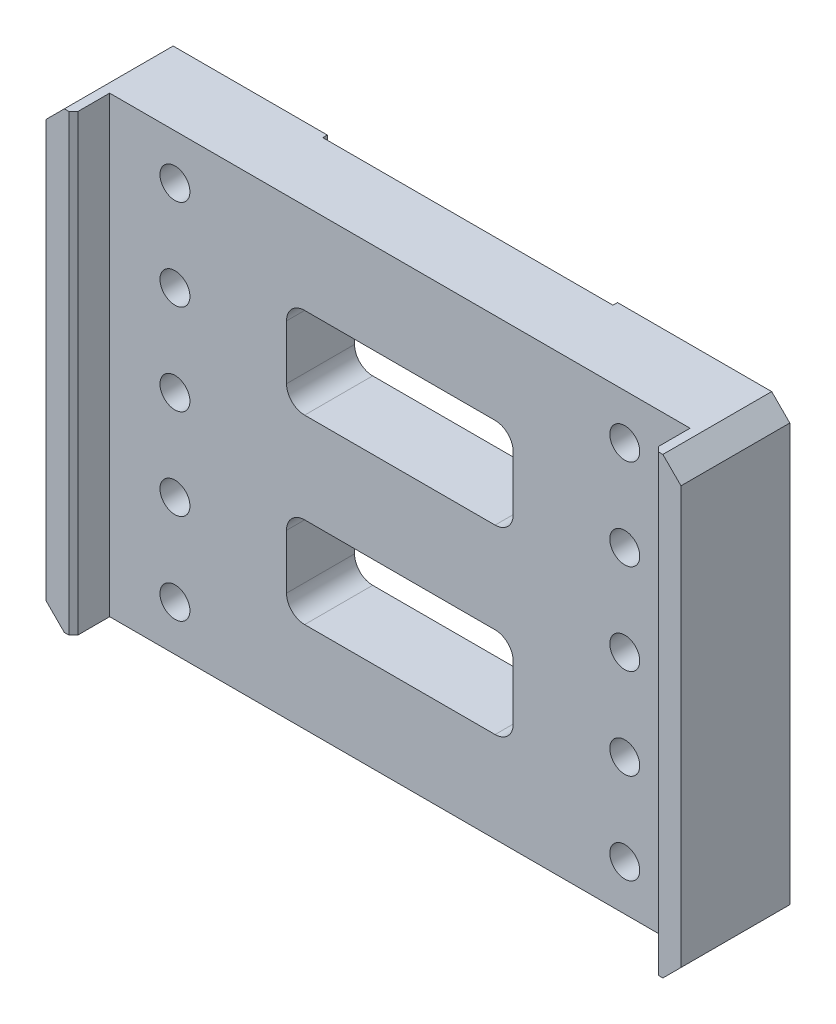
from build123d import *

# Parameters (mm, degrees)
SKETCH1_W           = 70
SKETCH1_H           = 50
BOSS_EXTRUDE1_DEPTH = 12
SKETCH2_W           = 64
SKETCH2_H           = 4
CUT_EXTRUDE1_DEPTH  = 63.20128616
CHAMFER1_SIZE       = 0.5
SKETCH3_W           = 32
SKETCH3_H           = 0.5
CUT_EXTRUDE2_DEPTH  = 63.20128616
LPATTERN1_COUNT     = 5
LPATTERN1_PITCH     = 10
SKETCH7_W           = 25
SKETCH7_H           = 10
CUT_EXTRUDE3_DEPTH  = 44.749285708
FILLET1_R           = 2
CHAMFER2_SIZE       = 2


with BuildPart() as part:
    # Sketch1 → Boss-Extrude1 (new body)
    with BuildSketch(Plane.XY):
        Rectangle(SKETCH1_W, SKETCH1_H)
    extrude(amount=BOSS_EXTRUDE1_DEPTH)

    # Sketch2 → Cut-Extrude1 (cut, through all)
    with BuildSketch(Plane.XZ.offset(25)):
        with Locations((0, 10)):
            Rectangle(SKETCH2_W, SKETCH2_H)
    extrude(amount=-CUT_EXTRUDE1_DEPTH, mode=Mode.SUBTRACT)

    # Chamfer1
    chamfer1_edges = [part.edges().sort_by_distance(p)[0] for p in [
        (-32, 0, 12),
        (32, 0, 12),
    ]]
    chamfer(chamfer1_edges, length=CHAMFER1_SIZE)

    # Sketch3 → Cut-Extrude2 (cut, through all)
    with BuildSketch(Plane(origin=(0, 25, 0), x_dir=(1, 0, 0), z_dir=(0, 1, 0))):
        with Locations((0, -0.25)):
            Rectangle(SKETCH3_W, SKETCH3_H)
    extrude(amount=-CUT_EXTRUDE2_DEPTH, mode=Mode.SUBTRACT)

    # Sketch6 → M4 Tapped Hole1 (revolve, cut)
    with BuildSketch(Plane(origin=(-24.8, 20, 8), x_dir=(0, -1, 0), z_dir=(1, 0, 0))):
        Polygon((0, 0), (0, 12.491420021), (1.65, 11.5), (1.65, 0), align=None)
    m4_tapped_hole1 = revolve(axis=Axis((-24.8, 20, 14.35), (0, 0, -1)), mode=Mode.SUBTRACT)

    # LPattern1: M4 Tapped Hole1 ×5
    with Locations(*[(0, -i * LPATTERN1_PITCH, 0) for i in range(1, LPATTERN1_COUNT)]):
        add(m4_tapped_hole1, mode=Mode.SUBTRACT)

    # Mirror1: M4 Tapped Hole1 across plane
    add(m4_tapped_hole1.mirror(Plane(origin=(0, 0, 0), x_dir=(0, 0, 1), z_dir=(1, 0, 0))), mode=Mode.SUBTRACT)

    # Mirror1 copy 1 sketch → Mirror1 copy 1 (revolve, cut)
    with BuildSketch(Plane(origin=(24.8, 10, 8), x_dir=(0, -1, 0), z_dir=(-1, 0, 0))):
        Polygon((0, 0), (0, -12.491420021), (1.65, -11.5), (1.65, 0), align=None)
    revolve(axis=Axis((24.8, 10, 14.35), (0, 0, 1)), mode=Mode.SUBTRACT)

    # Mirror1 copy 2 sketch → Mirror1 copy 2 (revolve, cut)
    with BuildSketch(Plane(origin=(24.8, 0, 8), x_dir=(0, -1, 0), z_dir=(-1, 0, 0))):
        Polygon((0, 0), (0, -12.491420021), (1.65, -11.5), (1.65, 0), align=None)
    revolve(axis=Axis((24.8, 0, 14.35), (0, 0, 1)), mode=Mode.SUBTRACT)

    # Mirror1 copy 3 sketch → Mirror1 copy 3 (revolve, cut)
    with BuildSketch(Plane(origin=(24.8, -10, 8), x_dir=(0, -1, 0), z_dir=(-1, 0, 0))):
        Polygon((0, 0), (0, -12.491420021), (1.65, -11.5), (1.65, 0), align=None)
    revolve(axis=Axis((24.8, -10, 14.35), (0, 0, 1)), mode=Mode.SUBTRACT)

    # Mirror1 copy 4 sketch → Mirror1 copy 4 (revolve, cut)
    with BuildSketch(Plane(origin=(24.8, -20, 8), x_dir=(0, -1, 0), z_dir=(-1, 0, 0))):
        Polygon((0, 0), (0, -12.491420021), (1.65, -11.5), (1.65, 0), align=None)
    revolve(axis=Axis((24.8, -20, 14.35), (0, 0, 1)), mode=Mode.SUBTRACT)

    # Sketch7 → Cut-Extrude3 (cut, through all)
    with BuildSketch(Plane.XY.offset(8)):
        with Locations((0, -10)):
            Rectangle(SKETCH7_W, SKETCH7_H)
        with Locations((0, 10)):
            Rectangle(SKETCH7_W, SKETCH7_H)
    extrude(amount=-CUT_EXTRUDE3_DEPTH, mode=Mode.SUBTRACT)

    # Fillet1
    fillet1_edges = [part.edges().sort_by_distance(p)[0] for p in [
        (-12.5, -15, 4.25),
        (-12.5, -5, 4.25),
        (12.5, -5, 4.25),
        (12.5, -15, 4.25),
        (12.5, 5, 4.25),
        (-12.5, 5, 4.25),
        (-12.5, 15, 4.25),
        (12.5, 15, 4.25),
    ]]
    fillet(fillet1_edges, radius=FILLET1_R)

    # Chamfer2
    chamfer2_edges = [part.edges().sort_by_distance(p)[0] for p in [
        (35, -25, 6),
        (-35, -25, 6),
        (-35, 25, 6),
        (35, 25, 6),
    ]]
    chamfer(chamfer2_edges, length=CHAMFER2_SIZE)


solid = part.part
